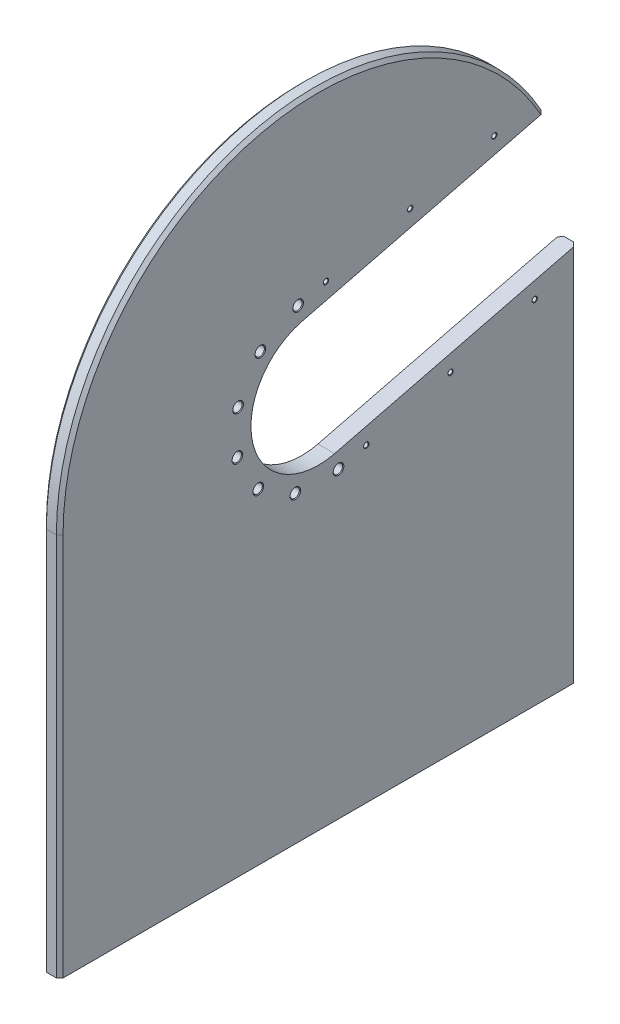
from build123d import *

# Parameters (mm, degrees)
BOSS_EXTRUDE1_DEPTH          = 25
CUT_EXTRUDE1_REACH           = 1039.876
M16_TAPPED_HOLE1_D           = 14
M16_TAPPED_HOLE1_CSINK_D     = 16.05
M16_TAPPED_HOLE1_CSINK_ANGLE = 90
CIRPATTERN1_COUNT            = 12
M8_TAPPED_HOLE1_D            = 6.8
M8_TAPPED_HOLE1_CSINK_D      = 8.05
M8_TAPPED_HOLE1_CSINK_ANGLE  = 90
LPATTERN1_COUNT              = 3
LPATTERN1_PITCH              = 130
MIRROR1_COPY_1_D             = 6.8
MIRROR1_COPY_1_CSINK_D       = 8.05
MIRROR1_COPY_1_CSINK_ANGLE   = 90
MIRROR1_COPY_2_D             = 6.8
MIRROR1_COPY_2_CSINK_D       = 8.05
MIRROR1_COPY_2_CSINK_ANGLE   = 90
CHAMFER1_SIZE                = 5


with BuildPart() as part:
    # Sketch1 → Boss-Extrude1 (new body)
    with BuildSketch(Plane(origin=(0, 0, 0), x_dir=(0, 0, -1), z_dir=(1, 0, 0))):
        with BuildLine():
            Line((-387.5, 575), (-387.5, 0))
            Line((-387.5, 0), (387.5, 0))
            Line((387.5, 0), (387.5, 575))
            ThreePointArc((387.5, 575), (0, 962.5), (-387.5, 575))
        make_face()
    extrude(amount=BOSS_EXTRUDE1_DEPTH)

    # Sketch2 → Cut-Extrude1 (cut, up to next)
    with BuildSketch(Plane(origin=(25, 0, 0), x_dir=(0, 0, -1), z_dir=(1, 0, 0)), mode=Mode.PRIVATE) as cut_extrude1_sk1:
        with BuildLine():
            Line((-24.434111456, 672.999868354), (338.559277668, 763.504285109))
            ThreePointArc((338.559277668, 763.504285109), (375.065307711, 672.37692207), (387.5, 575))
            Line((387.5, 575), (387.5, 567.522624537))
            Line((387.5, 567.522624537), (24.434111456, 477.000131646))
            ThreePointArc((24.434111456, 477.000131646), (-97.999868354, 550.565888544), (-24.434111456, 672.999868354))
        make_face()
    cut_extrude1_tool1 = extrude(cut_extrude1_sk1.sketch, amount=-CUT_EXTRUDE1_REACH, mode=Mode.PRIVATE) & part.part
    add(cut_extrude1_tool1.solids().sort_by_distance((25, 611.611981, -146.843429))[0], mode=Mode.SUBTRACT)

    # M16 Tapped Hole1 (through all)
    with Locations(Plane(origin=(25, 696.286965784, 30.24023695), x_dir=(0, 0, 1), z_dir=(1, 0, 0))):
        with Locations((0, 0)):
            m16_tapped_hole1 = CounterSinkHole(M16_TAPPED_HOLE1_D / 2, M16_TAPPED_HOLE1_CSINK_D / 2, counter_sink_angle=M16_TAPPED_HOLE1_CSINK_ANGLE)

    # CirPattern1: M16 Tapped Hole1 ×12 about axis, 5 skipped
    cirpattern1_axis = Axis((-0.001, 575, 0), (-1, 0, 0))
    add([m16_tapped_hole1.rotate(cirpattern1_axis, i * 360 / CIRPATTERN1_COUNT) for i in range(1, CIRPATTERN1_COUNT) if i not in (1, 2, 3, 4, 5)], mode=Mode.SUBTRACT)

    # M8 Tapped Hole1 (through all)
    with Locations(Plane(origin=(25, 706.689607295, -11.48247928), x_dir=(0, 0, 1), z_dir=(1, 0, 0))):
        with Locations((0, 0)):
            m8_tapped_hole1 = CounterSinkHole(M8_TAPPED_HOLE1_D / 2, M8_TAPPED_HOLE1_CSINK_D / 2, counter_sink_angle=M8_TAPPED_HOLE1_CSINK_ANGLE)

    # LPattern1: M8 Tapped Hole1 ×3
    with Locations(*[Vector(0, 0.24192189559966076, -0.9702957262759982) * (i * LPATTERN1_PITCH) for i in range(1, LPATTERN1_COUNT)]):
        add(m8_tapped_hole1, mode=Mode.SUBTRACT)

    # Mirror1: M8 Tapped Hole1 across plane
    add(m8_tapped_hole1.mirror(Plane(origin=(0, 541.347432947, 134.973074301), x_dir=(0, -0.24192189559966135, 0.970295726275998), z_dir=(0, 0.9702957262759981, 0.24192189559966135))), mode=Mode.SUBTRACT)

    # Mirror1 copy 1 (through all)
    with Locations(Plane(origin=(25, 495.565522155, -198.101397596), x_dir=(0, -0.4694715627858792, 0.8829475928589331), z_dir=(1, 0, 0))):
        with Locations((0, 0)):
            CounterSinkHole(MIRROR1_COPY_1_D / 2, MIRROR1_COPY_1_CSINK_D / 2, counter_sink_angle=MIRROR1_COPY_1_CSINK_ANGLE)

    # Mirror1 copy 2 (through all)
    with Locations(Plane(origin=(25, 527.015368582, -324.239842012), x_dir=(0, -0.4694715627858792, 0.8829475928589331), z_dir=(1, 0, 0))):
        with Locations((0, 0)):
            CounterSinkHole(MIRROR1_COPY_2_D / 2, MIRROR1_COPY_2_CSINK_D / 2, counter_sink_angle=MIRROR1_COPY_2_CSINK_ANGLE)

    # Chamfer1
    chamfer1_edges = [part.edges().sort_by_distance(p)[0] for p in [
        (0, 950.065307711, 97.37692207),
        (25, 950.065307711, 97.37692207),
        (25, 283.761312269, -387.5),
        (0, 283.761312269, -387.5),
        (0, 287.5, 387.5),
        (25, 287.5, 387.5),
    ]]
    chamfer(chamfer1_edges, length=CHAMFER1_SIZE)


solid = part.part
